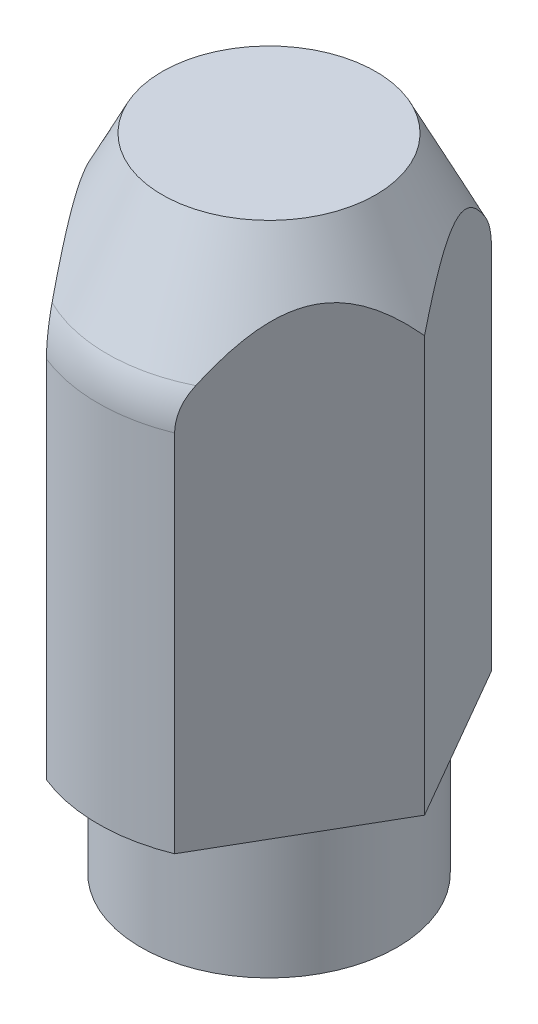
from build123d import *

# Parameters (mm, degrees)
M3_TAPPED_HOLE1_D     = 2.5
M3_TAPPED_HOLE1_DEPTH = 10
M3_TAPPED_HOLE1_TIP   = 0.751075774
CUT_EXTRUDE1_DEPTH    = 17.031219542
FILLET1_R             = 2


with BuildPart() as part:
    # Sketch1 → Revolve1 (revolve)
    with BuildSketch(Plane.XY):
        Polygon((0, 0), (0, 15), (2.5, 15), (4, 12), (4, 3), (3, 3), (3, 0), align=None)
    revolve(axis=Axis((0, 0, 0), (0, 1, 0)))

    # M3 Tapped Hole1
    with Locations(Plane(origin=(0, 0, 0), x_dir=(-1, 0, 0), z_dir=(0, -1, 0))):
        with Locations((0, 0)):
            Hole(M3_TAPPED_HOLE1_D / 2, depth=M3_TAPPED_HOLE1_DEPTH)
            with Locations((0, 0, -(M3_TAPPED_HOLE1_DEPTH + M3_TAPPED_HOLE1_TIP / 2))):  # 118° drill point
                Cone(0, M3_TAPPED_HOLE1_D / 2, M3_TAPPED_HOLE1_TIP, mode=Mode.SUBTRACT)

    # Sketch4 → Cut-Extrude1 (cut, through all)
    with BuildSketch(Plane(origin=(0, 15, 0), x_dir=(1, 0, 0), z_dir=(0, 1, 0))):
        with BuildLine():
            Line((-1.5, 3.708099244), (-3.640872096, 0))
            Line((-3.640872096, 0), (-1.5, -3.708099244))
            ThreePointArc((-1.5, -3.708099244), (-4, 0), (-1.5, 3.708099244))
        make_face()
        with BuildLine():
            Line((1.5, 3.708099244), (3.640872096, 0))
            Line((3.640872096, 0), (1.5, -3.708099244))
            ThreePointArc((1.5, -3.708099244), (4, 0), (1.5, 3.708099244))
        make_face()
    extrude(amount=-CUT_EXTRUDE1_DEPTH, mode=Mode.SUBTRACT)

    # Fillet1
    fillet1_edges = [part.edges().sort_by_distance(p)[0] for p in [
        (0, 12, -4),
        (0, 12, 4),
    ]]
    fillet(fillet1_edges, radius=FILLET1_R)


solid = part.part
